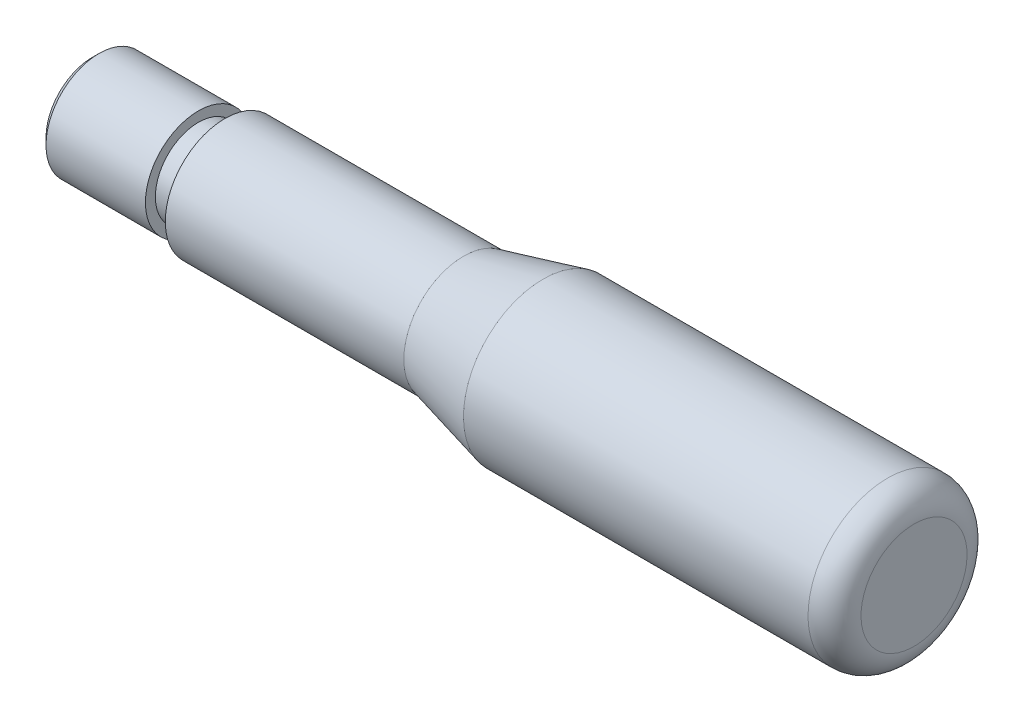
SolidWorks part; units mm, degrees
ref_plane "Front Plane" through (0, 0, 0) normal (0, 0, 1) x (1, 0, 0)
ref_plane "Top Plane" through (0, 0, 0) normal (0, 1, 0) x (1, 0, 0)
ref_plane "Right Plane" through (0, 0, 0) normal (1, 0, 0) x (0, 0, -1)
other "Configuration Table"
sketch "Sketch1" plane through (0, 0, 0) normal (0, 0, 1) x (1, 0, 0)
  line L0 (0, 0) -> (0, 4)
  line L1 (0, 4) -> (8, 4)
  line L2 (8, 4) -> (8, 3.25)
  line L3 (8, 3.25) -> (10, 3.25)
  line L4 (10, 3.25) -> (10, 4.5)
  line L5 (10, 4.5) -> (28, 4.5)
  line L6 (28, 4.5) -> (34, 6)
  line L7 (34, 6) -> (62, 6)
  line L8 (62, 6) -> (62, 0)
  line L9 (62, 0) -> (0, 0) construction
  line L10 (0, 0) -> (62, 0)
  dimension "D1" = 2
  dimension "D2" = 8
  dimension "D3" = 62
  dimension "D4" = 18
  dimension "D5" = 28
  dimension "D6" = 12
  dimension "D7" = 9
  dimension "D8" = 6.5
  dimension "D9" = 8
revolve "Revolve1" add sketch "Sketch1" angle 360 about L9
cosmetic thread "Cosmetic Thread1" parameters "D2"=6.647
fillet "Fillet1" radius 2 1 edges at (62, 6, 0)
chamfer "Chamfer1" distance 0.5 angle 45 1 edges at (0, 4, 0)
